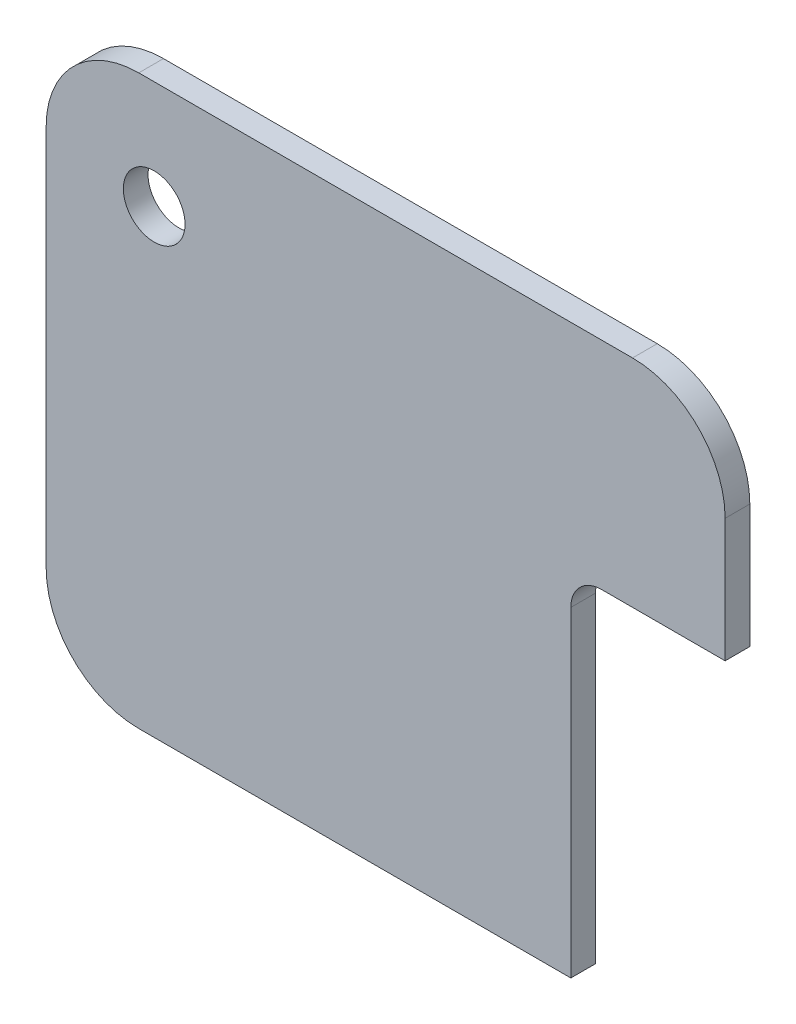
from build123d import *

# Parameters (mm, degrees)
SKETCH1_R           = 10
BOSS_EXTRUDE1_DEPTH = 8


with BuildPart() as part:
    # Sketch1 → Boss-Extrude1 (new body)
    with BuildSketch(Plane.XY):
        with BuildLine():
            Line((0, 30), (0, 154))
            ThreePointArc((0, 154), (8.786796564, 175.213203436), (30, 184))
            Line((30, 184), (190, 184))
            ThreePointArc((190, 184), (211.213203436, 175.213203436), (220, 154))
            Line((220, 154), (220, 114))
            Line((220, 114), (180, 114))
            ThreePointArc((180, 114), (172.928932188, 111.071067812), (170, 104))
            Line((170, 104), (170, 0))
            Line((170, 0), (30, 0))
            ThreePointArc((30, 0), (8.786796564, 8.786796564), (0, 30))
        make_face()
        with Locations((35, 149)):
            Circle(SKETCH1_R, mode=Mode.SUBTRACT)
    extrude(amount=BOSS_EXTRUDE1_DEPTH)


solid = part.part
